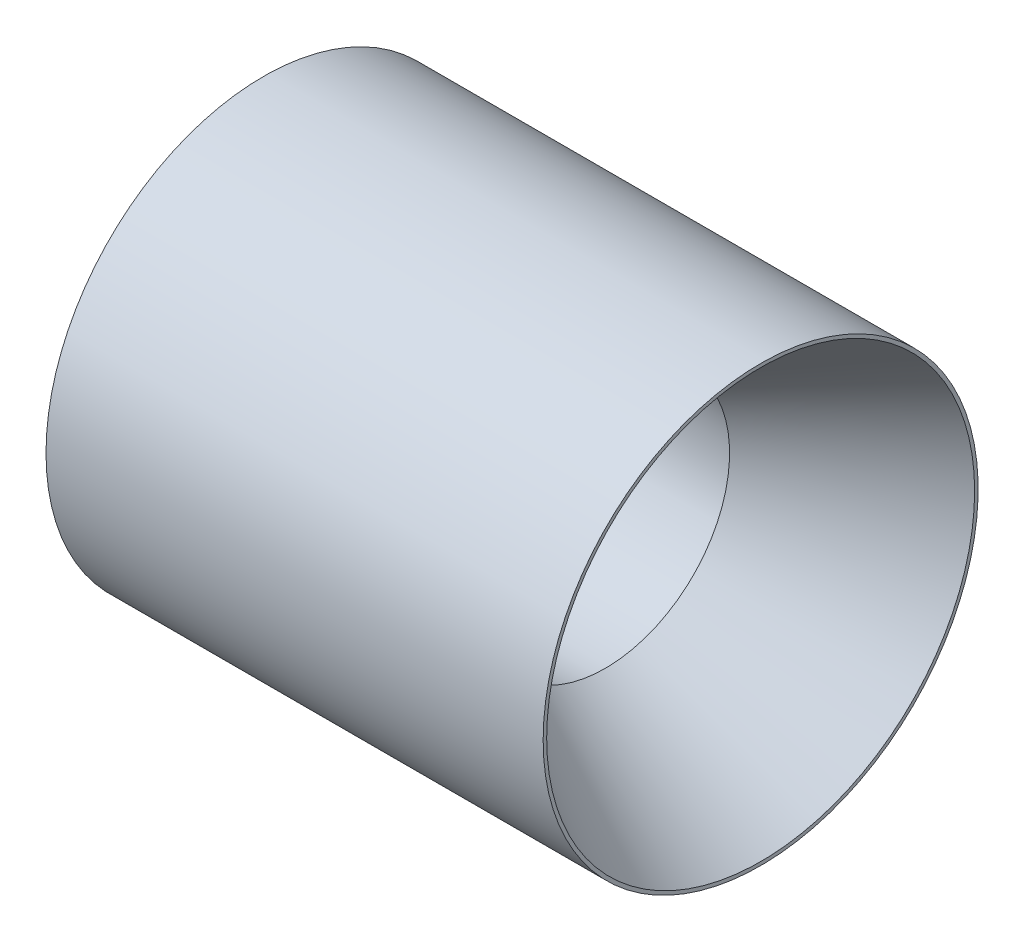
from build123d import *


with BuildPart() as part:
    # Sketch1 → Revolve1 (revolve)
    with BuildSketch(Plane.XY, mode=Mode.PRIVATE) as revolve1_sk:
        Polygon((0, 4), (11, 4), (16, 6.886751346), (16, 7), (0, 7), align=None)
    revolve(revolve1_sk.sketch.rotate(Axis((0, 0, 0), (1, 0, 0)), 90), axis=Axis((0, 0, 0), (1, 0, 0)))


solid = part.part
